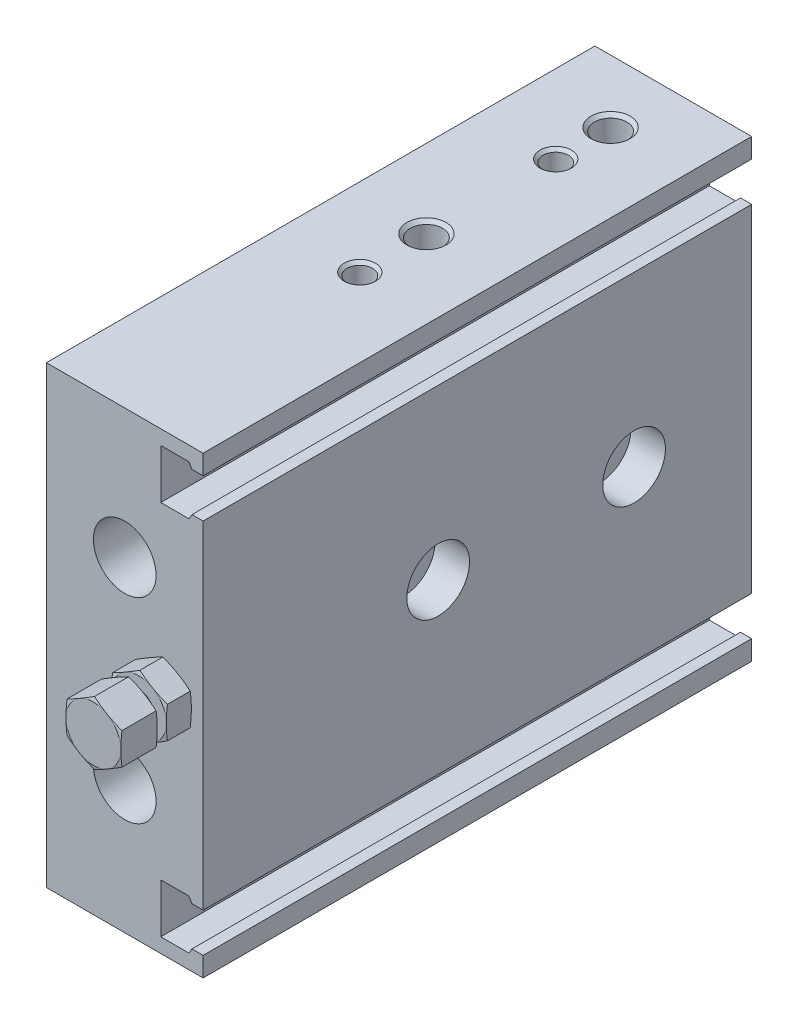
from build123d import *

# Parameters (mm, degrees)
BOSS_EXTRUDE1_DEPTH = 70
HOLE1_D             = 4.3
HOLE1_CBORE_D       = 8
HOLE1_CBORE_DEPTH   = 4.4
HOLE2_D             = 4.3
HOLE2_CBORE_D       = 8
HOLE2_CBORE_DEPTH   = 4.4
HOLE3_D             = 4.134
HOLE3_DEPTH         = 4.5
HOLE3_CSINK_D       = 5
HOLE3_CSINK_ANGLE   = 90
HOLE3_TIP           = 1.193383006
HOLE4_D             = 4.134
HOLE4_DEPTH         = 4.5
HOLE4_CSINK_D       = 5
HOLE4_CSINK_ANGLE   = 90
HOLE4_TIP           = 1.193383006
HOLE5_D             = 4.134
HOLE5_DEPTH         = 4.5
HOLE5_CSINK_D       = 5
HOLE5_CSINK_ANGLE   = 90
HOLE5_TIP           = 1.193383006
HOLE6_D             = 4.134
HOLE6_DEPTH         = 4.5
HOLE6_CSINK_D       = 5
HOLE6_CSINK_ANGLE   = 90
HOLE6_TIP           = 1.193383006
HOLE7_D             = 3.242
HOLE7_DEPTH         = 5
HOLE7_CSINK_D       = 4
HOLE7_CSINK_ANGLE   = 90
HOLE7_TIP           = 0.935884786
HOLE8_D             = 3.242
HOLE8_DEPTH         = 5
HOLE8_CSINK_D       = 4
HOLE8_CSINK_ANGLE   = 90
HOLE8_TIP           = 0.935884786
HOLE9_D             = 3.242
HOLE9_DEPTH         = 5
HOLE9_CSINK_D       = 4
HOLE9_CSINK_ANGLE   = 90
HOLE9_TIP           = 0.935884786
HOLE10_D            = 3.242
HOLE10_DEPTH        = 5
HOLE10_CSINK_D      = 4
HOLE10_CSINK_ANGLE  = 90
HOLE10_TIP          = 0.935884786
SKETCH28_R          = 8
CUT_EXTRUDE1_DEPTH  = 9


with BuildPart() as part:
    # Sketch1 → Boss-Extrude1 (new body)
    with BuildSketch(Plane.XY):
        Polygon((-10, 29), (-10, -29), (10, -29), (10, -26.5), (8.575277675, -26.5), (8.2, -27.15), (4.6, -27.15), (4.6, -20.85), (8.2, -20.85), (8.575277675, -21.5), (10, -21.5), (10, 21.5), (8.575277675, 21.5), (8.2, 20.85), (4.6, 20.85), (4.6, 27.15), (8.2, 27.15), (8.575277675, 26.5), (10, 26.5), (10, 29), align=None)
    extrude(amount=-BOSS_EXTRUDE1_DEPTH)

    # Sketch2 → Cut-Revolve1 (revolve, cut)
    with BuildSketch(Plane(origin=(0, 0, 0), x_dir=(0, 0, -1), z_dir=(1, 0, 0)), mode=Mode.PRIVATE) as cut_revolve1_sk:
        Polygon((0, 12.5), (0, 16.5), (30, 16.5), (30, 20), (45, 20), (45, 12.5), align=None)
    revolve(cut_revolve1_sk.sketch.rotate(Axis((0, 12.5, -45), (0, 0, 1)), 270), axis=Axis((0, 12.5, -45), (0, 0, 1)), mode=Mode.SUBTRACT)

    # Sketch3 → Cut-Revolve2 (revolve, cut)
    with BuildSketch(Plane(origin=(0, 0, 0), x_dir=(0, 0, -1), z_dir=(1, 0, 0)), mode=Mode.PRIVATE) as cut_revolve2_sk:
        Polygon((0, -12.5), (0, -8.5), (30, -8.5), (30, -5), (45, -5), (45, -12.5), align=None)
    revolve(cut_revolve2_sk.sketch.rotate(Axis((0, -12.5, -45), (0, 0, 1)), 270), axis=Axis((0, -12.5, -45), (0, 0, 1)), mode=Mode.SUBTRACT)

    # Hole1 (through all)
    with Locations(Plane(origin=(10, 0, 0), x_dir=(0, 0, -1), z_dir=(1, 0, 0))):
        with Locations((30, 0)):
            CounterBoreHole(HOLE1_D / 2, HOLE1_CBORE_D / 2, HOLE1_CBORE_DEPTH)

    # Hole2 (through all)
    with Locations(Plane(origin=(10, 0, 0), x_dir=(0, 0, -1), z_dir=(1, 0, 0))):
        with Locations((55, 0)):
            CounterBoreHole(HOLE2_D / 2, HOLE2_CBORE_D / 2, HOLE2_CBORE_DEPTH)

    # Sketch8 → Cut-Revolve3 (revolve, cut)
    with BuildSketch(Plane.XY.offset(-30), mode=Mode.PRIVATE) as cut_revolve3_sk:
        Polygon((-10, 0), (-10, 2.5), (-9.567, 2.067), (-2, 2.067), (-0.806616994, 0), align=None)
    revolve(cut_revolve3_sk.sketch.rotate(Axis((-0.806616994, 0, -30), (-1, 0, 0)), 90), axis=Axis((-0.806616994, 0, -30), (-1, 0, 0)), mode=Mode.SUBTRACT)

    # Sketch9 → Cut-Revolve4 (revolve, cut)
    with BuildSketch(Plane.XY.offset(-55), mode=Mode.PRIVATE) as cut_revolve4_sk:
        Polygon((-10, 0), (-10, 2.5), (-9.567, 2.067), (-2, 2.067), (-0.806616994, 0), align=None)
    revolve(cut_revolve4_sk.sketch.rotate(Axis((-0.806616994, 0, -55), (-1, 0, 0)), 90), axis=Axis((-0.806616994, 0, -55), (-1, 0, 0)), mode=Mode.SUBTRACT)

    # Hole3
    with Locations(Plane(origin=(0, 29, 0), x_dir=(1, 0, 0), z_dir=(0, 1, 0))):
        with Locations((0, 38.5)):
            CounterSinkHole(HOLE3_D / 2, HOLE3_CSINK_D / 2, depth=HOLE3_DEPTH, counter_sink_angle=HOLE3_CSINK_ANGLE)
            with Locations((0, 0, -(HOLE3_DEPTH + HOLE3_TIP / 2))):  # 120° drill point
                Cone(0, HOLE3_D / 2, HOLE3_TIP, mode=Mode.SUBTRACT)

    # Hole4
    with Locations(Plane(origin=(0, 29, 0), x_dir=(1, 0, 0), z_dir=(0, 1, 0))):
        with Locations((0, 62)):
            CounterSinkHole(HOLE4_D / 2, HOLE4_CSINK_D / 2, depth=HOLE4_DEPTH, counter_sink_angle=HOLE4_CSINK_ANGLE)
            with Locations((0, 0, -(HOLE4_DEPTH + HOLE4_TIP / 2))):  # 120° drill point
                Cone(0, HOLE4_D / 2, HOLE4_TIP, mode=Mode.SUBTRACT)

    # Hole5
    with Locations(Plane(origin=(0, -29, 0), x_dir=(-1, 0, 0), z_dir=(0, -1, 0))):
        with Locations((0, 38.5)):
            CounterSinkHole(HOLE5_D / 2, HOLE5_CSINK_D / 2, depth=HOLE5_DEPTH, counter_sink_angle=HOLE5_CSINK_ANGLE)
            with Locations((0, 0, -(HOLE5_DEPTH + HOLE5_TIP / 2))):  # 120° drill point
                Cone(0, HOLE5_D / 2, HOLE5_TIP, mode=Mode.SUBTRACT)

    # Hole6
    with Locations(Plane(origin=(0, -29, 0), x_dir=(-1, 0, 0), z_dir=(0, -1, 0))):
        with Locations((0, 62)):
            CounterSinkHole(HOLE6_D / 2, HOLE6_CSINK_D / 2, depth=HOLE6_DEPTH, counter_sink_angle=HOLE6_CSINK_ANGLE)
            with Locations((0, 0, -(HOLE6_DEPTH + HOLE6_TIP / 2))):  # 120° drill point
                Cone(0, HOLE6_D / 2, HOLE6_TIP, mode=Mode.SUBTRACT)

    # Hole7
    with Locations(Plane(origin=(0, 29, 0), x_dir=(1, 0, 0), z_dir=(0, 1, 0))):
        with Locations((0, 30)):
            CounterSinkHole(HOLE7_D / 2, HOLE7_CSINK_D / 2, depth=HOLE7_DEPTH, counter_sink_angle=HOLE7_CSINK_ANGLE)
            with Locations((0, 0, -(HOLE7_DEPTH + HOLE7_TIP / 2))):  # 120° drill point
                Cone(0, HOLE7_D / 2, HOLE7_TIP, mode=Mode.SUBTRACT)

    # Hole8
    with Locations(Plane(origin=(0, 29, 0), x_dir=(1, 0, 0), z_dir=(0, 1, 0))):
        with Locations((0, 55)):
            CounterSinkHole(HOLE8_D / 2, HOLE8_CSINK_D / 2, depth=HOLE8_DEPTH, counter_sink_angle=HOLE8_CSINK_ANGLE)
            with Locations((0, 0, -(HOLE8_DEPTH + HOLE8_TIP / 2))):  # 120° drill point
                Cone(0, HOLE8_D / 2, HOLE8_TIP, mode=Mode.SUBTRACT)

    # Hole9
    with Locations(Plane(origin=(0, -29, 0), x_dir=(-1, 0, 0), z_dir=(0, -1, 0))):
        with Locations((0, 30)):
            CounterSinkHole(HOLE9_D / 2, HOLE9_CSINK_D / 2, depth=HOLE9_DEPTH, counter_sink_angle=HOLE9_CSINK_ANGLE)
            with Locations((0, 0, -(HOLE9_DEPTH + HOLE9_TIP / 2))):  # 120° drill point
                Cone(0, HOLE9_D / 2, HOLE9_TIP, mode=Mode.SUBTRACT)

    # Hole10
    with Locations(Plane(origin=(0, -29, 0), x_dir=(-1, 0, 0), z_dir=(0, -1, 0))):
        with Locations((0, 55)):
            CounterSinkHole(HOLE10_D / 2, HOLE10_CSINK_D / 2, depth=HOLE10_DEPTH, counter_sink_angle=HOLE10_CSINK_ANGLE)
            with Locations((0, 0, -(HOLE10_DEPTH + HOLE10_TIP / 2))):  # 120° drill point
                Cone(0, HOLE10_D / 2, HOLE10_TIP, mode=Mode.SUBTRACT)

    # Sketch26 → Revolve1 (revolve)
    with BuildSketch(Plane(origin=(5, 0, 0), x_dir=(0, 0, -1), z_dir=(1, 0, 0)), mode=Mode.PRIVATE) as revolve1_sk:
        Polygon((-3.2, 0), (-3.2, 3.5), (-2.262177826, 7), (-0.937822174, 7), (0, 3.5), (0, 0), align=None)
    revolve(revolve1_sk.sketch.rotate(Axis((5, 0, 0), (0, 0, 1)), 270), axis=Axis((5, 0, 0), (0, 0, 1)))

    # Sketch27 → Revolve2 (revolve)
    with BuildSketch(Plane(origin=(5, 0, 0), x_dir=(0, 0, -1), z_dir=(1, 0, 0)), mode=Mode.PRIVATE) as revolve2_sk:
        Polygon((-9, 0), (-9, 3.5), (-8.062177826, 7), (-5.287822174, 7), (-4.35, 3.5), (-4.35, 2), (-3.2, 2), (-3.2, 0), align=None)
    revolve(revolve2_sk.sketch.rotate(Axis((5, 0, 3.2), (0, 0, 1)), 270), axis=Axis((5, 0, 3.2), (0, 0, 1)))

    # Sketch28 → Cut-Extrude1 (cut)
    with BuildSketch(Plane.XY):
        with Locations((5, 0)):
            Circle(SKETCH28_R)
        Polygon((1.5, 2.020725942), (1.5, -2.020725942), (5, -4.041451884), (8.5, -2.020725942), (8.5, 2.020725942), (5, 4.041451884), align=None, mode=Mode.SUBTRACT)
    extrude(amount=CUT_EXTRUDE1_DEPTH, mode=Mode.SUBTRACT)


solid = part.part
